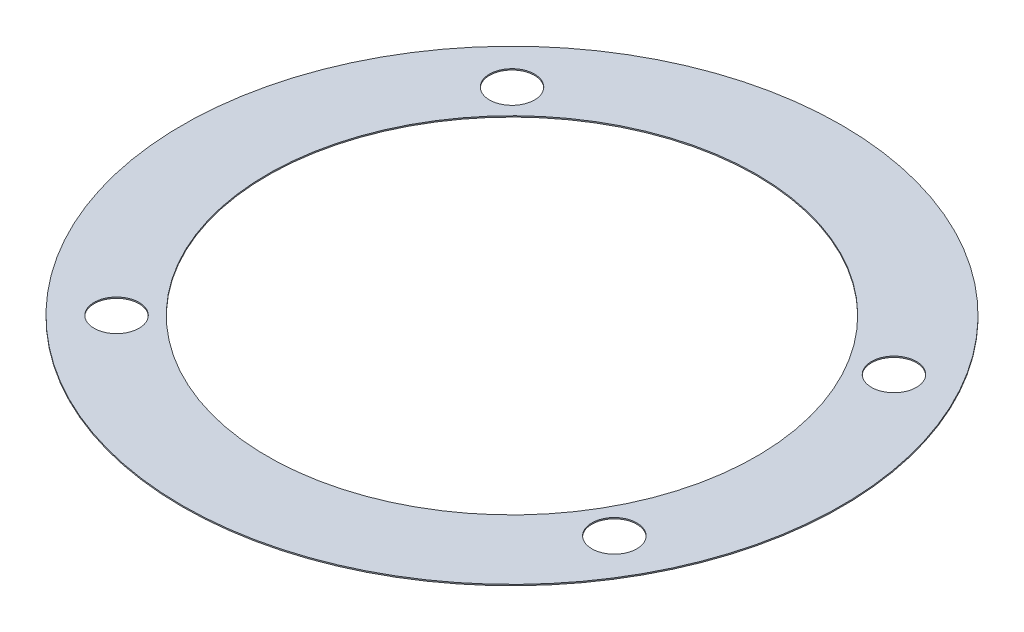
from build123d import *

# Parameters (mm, degrees)
SKETCH1_R                               = 104.775
SKETCH1_R_2                             = 77.724
BOSS_EXTRUDE1_DEPTH                     = 0.381
F_9_16_0_5625_DIAMETER_HOLE1_AT_2_COUNT = 2
F_9_16_0_5625_DIAMETER_HOLE1_AT_2_PITCH = 141.053237967


with BuildPart() as part:
    # Sketch1 → Boss-Extrude1 (new body)
    with BuildSketch(Plane(origin=(0, 0, 0), x_dir=(1, 0, 0), z_dir=(0, 1, 0))):
        with Locations(Location((0, 0, 0), (0, 0, 90))):
            Circle(SKETCH1_R)
        with Locations(Location((0, 0, 0), (0, 0, 90))):
            Circle(SKETCH1_R_2, mode=Mode.SUBTRACT)
    extrude(amount=BOSS_EXTRUDE1_DEPTH)

    # Sketch2 → 9/16 (0.5625) Diameter Hole1 (revolve, cut)
    with BuildSketch(Plane(origin=(-62.8586, 0.381, -62.865), x_dir=(0, 0, 1), z_dir=(1, 0, 0))):
        Polygon((0, 0), (0, 20.172398047), (7.14375, 15.88), (7.14375, 0), align=None)
    f_9_16_0_5625_diameter_hole1 = revolve(axis=Axis((-62.8586, 6.731, -62.865), (0, -1, 0)), mode=Mode.SUBTRACT)

    # 9/16 (0.5625) Diameter Hole1 at 2: 9/16 (0.5625) Diameter Hole1 ×2
    with Locations(*[Vector(0.9914412601618559, 0, 0.1305535432252662) * (i * F_9_16_0_5625_DIAMETER_HOLE1_AT_2_PITCH) for i in range(1, F_9_16_0_5625_DIAMETER_HOLE1_AT_2_COUNT)]):
        add(f_9_16_0_5625_diameter_hole1, mode=Mode.SUBTRACT)

    # Mirror1: 9/16 (0.5625) Diameter Hole1 across plane
    add(f_9_16_0_5625_diameter_hole1.mirror(Plane.XY), mode=Mode.SUBTRACT)

    # Mirror1 copy 1 sketch → Mirror1 copy 1 (revolve, cut)
    with BuildSketch(Plane(origin=(76.9874, 0.381, 44.45), x_dir=(0, 0, -1), z_dir=(1, 0, 0))):
        Polygon((0, 0), (0, -20.172398047), (7.14375, -15.88), (7.14375, 0), align=None)
    revolve(axis=Axis((76.9874, 6.731, 44.45), (0, 1, 0)), mode=Mode.SUBTRACT)


solid = part.part
